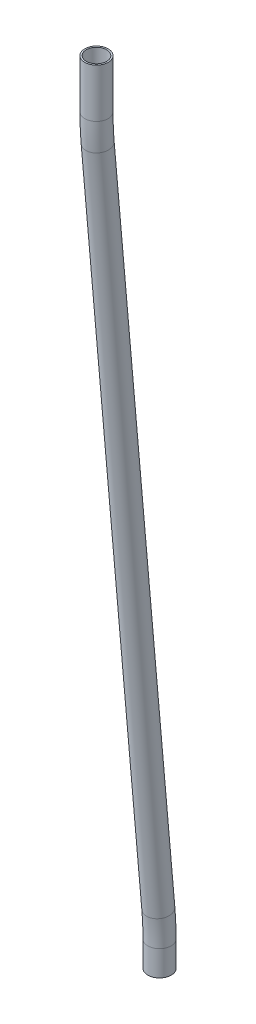
from build123d import *

# Parameters (mm, degrees)
SWEEP_THIN1_PROFILE_R   = 15
SWEEP_THIN1_PROFILE_R_2 = 13


with BuildPart() as part:
    # Sweep-Thin1: sweep along a curve in space
    with BuildLine() as sweep_thin1_path:
        Line((19403.083026604, -840, -3659.86490803), (19403.083026604, -807.464377163, -3659.86490803))
        ThreePointArc((19403.083026604, -807.464377163, -3659.86490803), (19403.083026604, -790.016622217, -3659.484196663), (19403.083026604, -772.602080064, -3658.342787267))
        Line((19403.083026604, -772.602080064, -3658.342787267), (19403.083026604, 116.074565195, -3580.593655266))
        ThreePointArc((19403.083026604, 116.074565195, -3580.593655266), (19403.083026604, 133.489107348, -3579.45224587), (19403.083026604, 150.936862294, -3579.071534503))
        Line((19403.083026604, 150.936862294, -3579.071534503), (19403.083026604, 213.472485131, -3579.071534503))
    # Sweep-Thin1 profile (on start of the path) → Sweep-Thin1 (sweep)
    with BuildSketch(Plane(origin=(19403.083026604, -840, -3659.86490803), x_dir=(0, 0, 1), z_dir=(0, 1, 0))):
        Circle(SWEEP_THIN1_PROFILE_R)
        Circle(SWEEP_THIN1_PROFILE_R_2, mode=Mode.SUBTRACT)
    sweep(path=sweep_thin1_path.line)


solid = part.part
